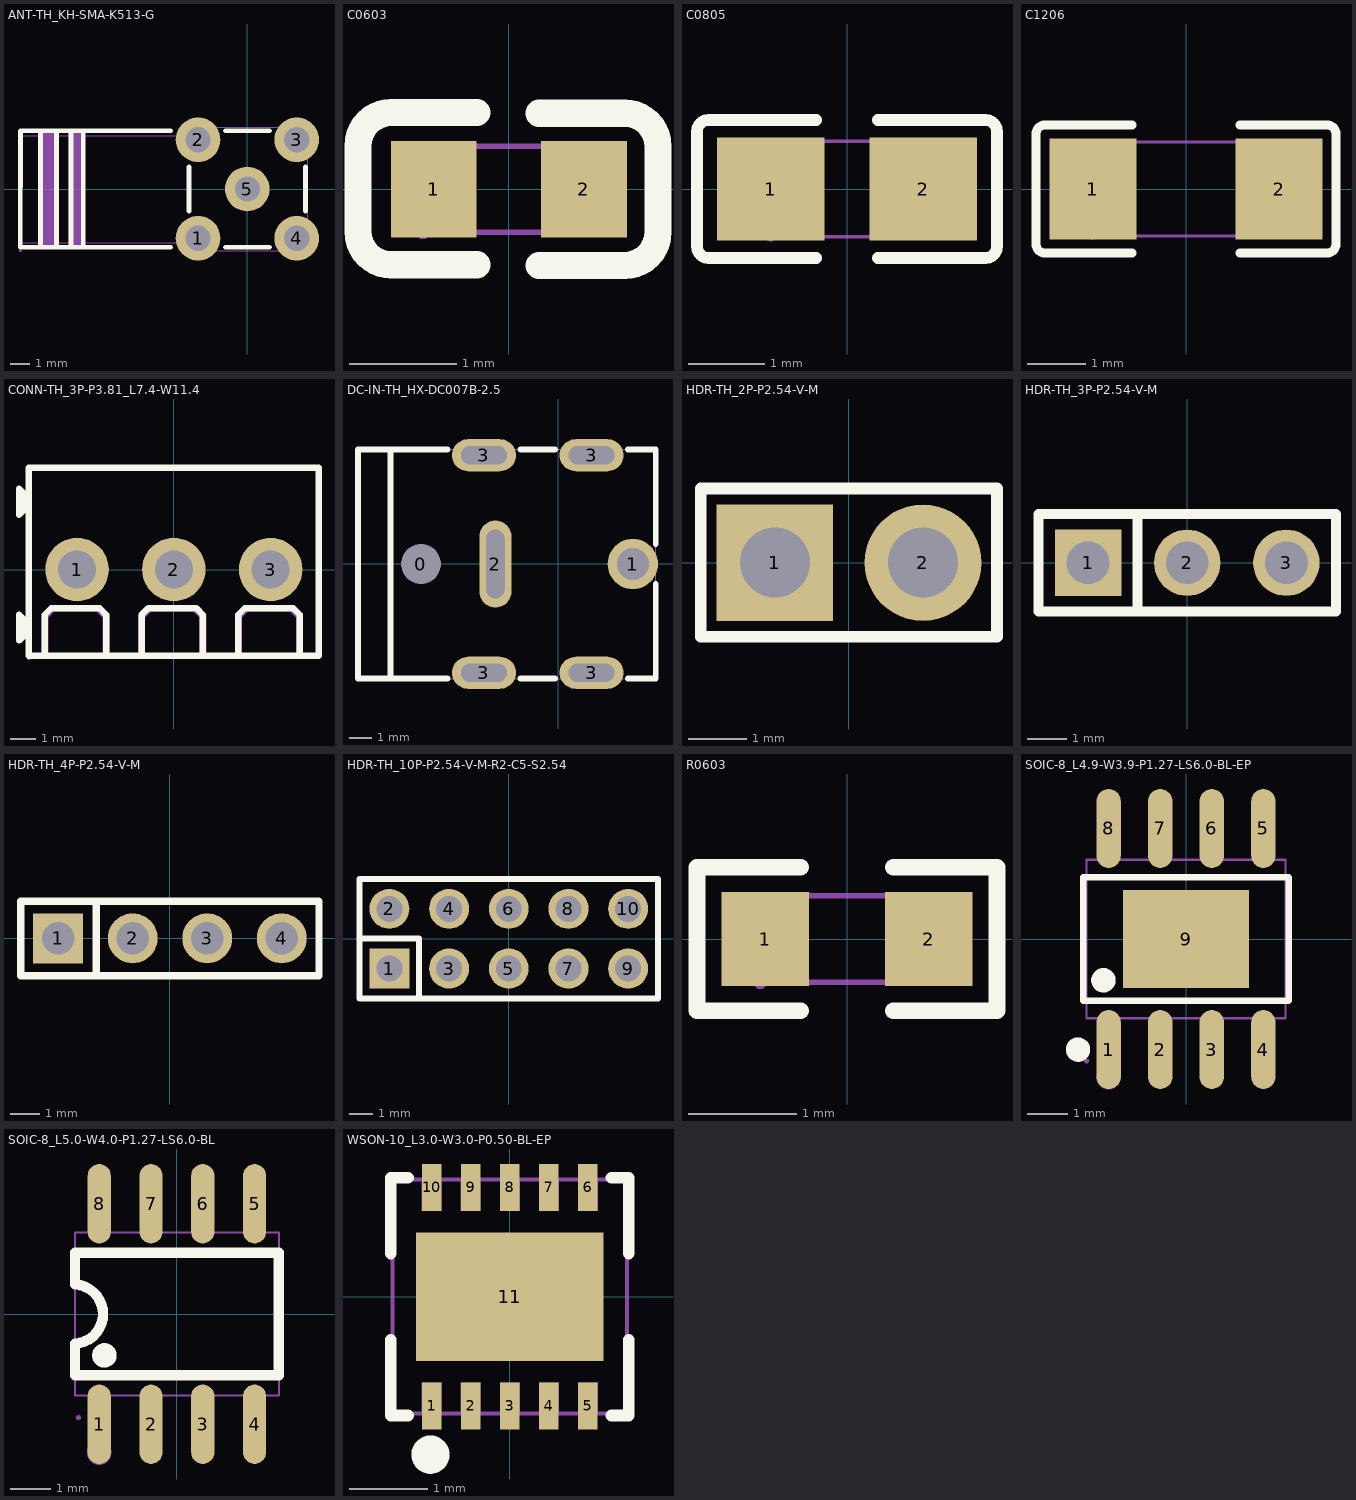
[diagram p0: the footprints below, top view; thin cyan lines are the x and y axes]
# Altium footprint library MISC75514-5.PcbLib: 14 footprints
Each footprint in its own frame and in the unit in brackets; x right, y up, seen from the top. Pads: shape width x height; smd on the part's side, far side on the other; paste and mask are expansions set on the pad; w line width, h text height; cw(c..) or ccw(c..) is an arc to the next point about the centre after c.

## ANT-TH_KH-SMA-K513-G [mm]
height 1.4
pads (5):
  round 2.3 hole 1.3 paste+0.051: 1(-2.54,-2.54) 2(-2.54,2.54) 3(2.54,2.54) 4(2.54,-2.54) 5(0,0)
Top Overlay:
  lines w0.254: -11.69,2.98 -11.7,-2.83 -11.7,-3 -11.5,-3 -3.948,-3 ; -11.69,3 -11.361,3 ; -11.5,3 -3.948,3 ; -10.668,-3 -10.668,3 ; -9.966,3 -9.573,3 ; -9.827,-3 -9.827,3 ; -9.09,-3 -9.09,3 ; -8.595,3 -8.176,3 ; -8.455,-3 -8.455,3 ; -3,-1.132 -3,1.132 ; -1.132,-3 1.132,-3 ; -1.132,3 1.132,3 ; 3,-1.132 3,1.132
Mechanical 2:
  region: -10.64,3 -9.84,3 -9.84,-2.99 -9.85,-3 -10.65,-3
  region: -9.194,2.972 -8.394,2.972 -8.394,-3.018 -8.404,-3.028 -9.204,-3.028
Mechanical 6:
  lines w0.051: -11.7,-2.76 -11.7,2.75 -3.25,2.75 -3.25,3.17 3.1,3.17 3.1,-3.18 -3.25,-3.17 -3.25,-2.76 -11.7,-2.76
Mechanical 8:
  region: -11.635,-3.18 -11.654,-3.226 -11.7,-3.245 -11.746,-3.226 -11.765,-3.18 -11.746,-3.134 -11.7,-3.115 -11.654,-3.134
Mechanical 9:
  region: 0.408,0 0.377,-0.156 0.288,-0.288 0.156,-0.377 0,-0.408 -0.156,-0.377 -0.288,-0.288 -0.377,-0.156 -0.408,0 -0.377,0.156 -0.288,0.288 -0.156,0.377 0,0.408 0.156,0.377 0.288,0.288 0.377,0.156
  region: 2.09,-2.09 2.99,-2.09 2.99,-2.99 2.09,-2.99
  region: -2.99,2.99 -2.09,2.99 -2.09,2.09 -2.99,2.09
  region: 2.09,2.99 2.99,2.99 2.99,2.09 2.09,2.09
  region: -2.99,-2.09 -2.09,-2.09 -2.09,-2.99 -2.99,-2.99

## C0603 [mm]
height 1.4
pads (2):
  rect 0.8x0.9 smd: 1(-0.7,0) 2(0.7,0)
Top Overlay:
  lines w0.254: -0.296,-0.704 -1.096,-0.704 cw(c-1.096,-0.394) -1.406,-0.394 -1.405,0.406 cw(c-1.096,0.406) -1.096,0.715 -0.296,0.715 ; 0.28,-0.71 1.08,-0.71 ccw(c1.08,-0.4) 1.39,-0.4 1.39,0.4 ccw(c1.08,0.4) 1.08,0.71 0.28,0.71
Mechanical 15:
  region: -0.74,-0.4 -0.74,-0.375 -0.775,-0.341 -0.825,-0.341 -0.86,-0.375 -0.86,-0.4 -0.86,-0.425 -0.825,-0.459 -0.776,-0.459 -0.741,-0.425 -0.74,-0.4
  region: 0.8,-0.4 0.8,0.4 0.5,0.4 0.5,-0.4
  region: -0.8,-0.4 -0.8,0.4 -0.5,0.4 -0.5,-0.4
  lines w0.051: -0.8,-0.4 0.8,-0.4 0.8,0.4 -0.8,0.4 -0.8,-0.4

## C0805 [mm]
height 1.4
pads (2):
  rect 1.41x1.35 smd paste-100 mask+0.051: 1(-1,0) 2(1,0)
Top Overlay:
  lines w0.152: -0.401,-0.904 -1.811,-0.904 cw(c-1.811,-0.751) -1.964,-0.751 -1.964,0.751 cw(c-1.811,0.751) -1.811,0.904 -0.401,0.904 ; 0.401,-0.904 1.811,-0.904 ccw(c1.811,-0.751) 1.964,-0.751 1.964,0.751 ccw(c1.811,0.751) 1.811,0.904 0.401,0.904
Top Paste:
  region: 1.705,0.64 1.705,-0.64 1.655,-0.69 0.505,-0.69 0.455,-0.64 0.45,-0.23 0.9,-0.23 0.9,0.22 0.46,0.22 0.455,0.64 0.505,0.69 1.655,0.69
  region: -1.705,-0.64 -1.705,0.64 -1.655,0.69 -0.505,0.69 -0.455,0.64 -0.45,0.23 -0.9,0.23 -0.9,-0.22 -0.46,-0.22 -0.455,-0.64 -0.505,-0.69 -1.655,-0.69
Mechanical 6:
  lines w0.051: -1,-0.625 1,-0.625 1,0.625 -1,0.625 -1,-0.625
Mechanical 8:
  region: -0.935,-0.625 -0.954,-0.671 -1,-0.69 -1.046,-0.671 -1.065,-0.625 -1.046,-0.579 -1,-0.56 -0.954,-0.579
Mechanical 9:
  region: 1,0.625 1,-0.625 0.5,-0.625 0.5,0.625
  region: -1,-0.625 -1,0.625 -0.5,0.625 -0.5,-0.625

## C1206 [mm]
height 1.4
pads (2):
  rect 1.485x1.728 smd paste-100 mask+0.051: 1(-1.593,0) 2(1.593,0)
Top Overlay:
  lines w0.152: -0.926,-1.093 -2.411,-1.093 cw(c-2.411,-0.94) -2.564,-0.94 -2.564,0.94 cw(c-2.411,0.94) -2.411,1.093 -0.926,1.093 ; 0.926,-1.093 2.411,-1.093 ccw(c2.411,-0.94) 2.564,-0.94 2.564,0.94 ccw(c2.411,0.94) 2.411,1.093 0.926,1.093
Top Paste:
  region: -0.85,-0.764 -0.85,-0.394 -0.95,-0.294 -1.255,-0.294 -1.355,-0.194 -1.355,0.194 -1.255,0.294 -0.95,0.294 -0.85,0.394 -0.85,0.764 -0.95,0.864 -2.235,0.864 -2.335,0.764 -2.335,-0.764 -2.235,-0.864 -0.95,-0.864
  region: 0.85,-0.764 0.85,-0.394 0.95,-0.294 1.255,-0.294 1.355,-0.194 1.355,0.194 1.255,0.294 0.95,0.294 0.85,0.394 0.85,0.764 0.95,0.864 2.235,0.864 2.335,0.764 2.335,-0.764 2.235,-0.864 0.95,-0.864
Mechanical 6:
  lines w0.051: -1.6,-0.8 1.6,-0.8 1.6,0.8 -1.6,0.8 -1.6,-0.8
Mechanical 8:
  region: -1.535,-0.8 -1.554,-0.846 -1.6,-0.865 -1.646,-0.846 -1.665,-0.8 -1.646,-0.754 -1.6,-0.735 -1.554,-0.754
Mechanical 9:
  region: 1.6,-0.8 1.6,0.8 1.1,0.8 1.1,-0.8
  region: -1.6,-0.8 -1.6,0.8 -1.1,0.8 -1.1,-0.8

## CONN-TH_3P-P3.81_L7.4-W11.4 [mm]
height 1.4
pads (3):
  round 2.5 hole 1.5 paste+0.051: 1(-3.81,0) 2(0,0) 3(3.81,0)
Top Overlay:
  region: -5.715,2.921 -5.842,2.921 -6.096,3.175 -6.096,2.286 -5.969,2.286 -5.715,2.54
  region: -5.651,-2.095 -5.778,-2.095 -6.032,-1.841 -6.032,-2.73 -5.905,-2.73 -5.651,-2.476
  lines w0.254: -5.715,-2.54 -5.842,-2.54 -6.096,-2.794 -6.096,-1.778 -5.842,-2.032 -5.715,-2.032 ; -5.715,2.413 -5.842,2.413 -6.096,2.159 -6.096,3.175 -5.842,2.921 -5.715,2.921 ; -5.08,-3.302 -5.08,-1.778 -4.826,-1.524 -2.921,-1.524 -2.667,-1.778 -2.667,-3.302 ; -1.27,-3.302 -1.27,-1.778 -1.016,-1.524 0.889,-1.524 1.143,-1.778 1.143,-3.302 ; 2.54,-3.302 2.54,-1.778 2.794,-1.524 4.699,-1.524 4.953,-1.778 4.953,-3.302 ; -5.71,-3.4 5.71,-3.4 5.71,4 -5.71,4 -5.71,-3.4
Mechanical 2:
  region: -5.207,-3.429 -5.207,-1.778 -4.826,-1.397 -2.921,-1.397 -2.54,-1.778 -2.54,-3.429 -2.794,-3.429 -2.794,-1.905 -3.048,-1.651 -4.699,-1.651 -4.953,-1.905 -4.953,-3.429
  region: -1.397,-3.429 -1.397,-1.778 -1.016,-1.397 0.889,-1.397 1.27,-1.778 1.27,-3.429 1.016,-3.429 1.016,-1.905 0.762,-1.651 -0.889,-1.651 -1.143,-1.905 -1.143,-3.429
  region: 2.413,-3.429 2.413,-1.778 2.794,-1.397 4.699,-1.397 5.08,-1.778 5.08,-3.429 4.826,-3.429 4.826,-1.905 4.572,-1.651 2.921,-1.651 2.667,-1.905 2.667,-3.429
Mechanical 6:
  lines w0.051: -5.715,-3.5 -5.715,3.9 5.715,3.9 5.715,-3.5 -5.715,-3.5
Mechanical 8:
  region: -5.65,-3.5 -5.669,-3.546 -5.715,-3.565 -5.761,-3.546 -5.78,-3.5 -5.761,-3.454 -5.715,-3.435 -5.669,-3.454
Mechanical 9:
  region: 3.36,0.3 4.26,0.3 4.26,-0.3 3.36,-0.3
  region: -0.45,0.3 0.45,0.3 0.45,-0.3 -0.45,-0.3
  region: -4.26,0.3 -3.36,0.3 -3.36,-0.3 -4.26,-0.3

## DC-IN-TH_HX-DC007B-2.5 [mm]
height 1.4
pads (7):
  round 1.7 hole 1.7 unplated: 0(-6,0)
  round 2.2 hole 1.4: 1(3.25,0)
  oval 1.4x3.8 hole 0.8 slot 3 at 90 deg: 2(-2.75,0)
  oval 2.8x1.4 hole 0.8 slot 2 at 0 deg: 3(-3.25,-4.75) 3(-3.25,4.75) 3(1.45,-4.75) 3(1.45,4.75)
Top Overlay:
  lines w0.254: -7.325,-5 -7.325,5 ; -4.847,-5 -8.75,-5 -8.75,5 -4.847,5 ; -1.653,-5 -0.147,-5 ; -1.653,5 -0.147,5 ; 3.047,-5 4.25,-5 4.25,-0.877 ; 3.047,5 4.25,5 4.25,0.877
Mechanical 1:
  circle w0.005: c-6,0 r0.85
Mechanical 15:
  region: 3.85,0 3.85,0.119 3.759,0.34 3.59,0.509 3.369,0.6 3.131,0.6 2.91,0.509 2.741,0.34 2.65,0.119 2.65,0 2.65,-0.119 2.741,-0.34 2.91,-0.509 3.131,-0.6 3.369,-0.6 3.59,-0.509 3.759,-0.34 3.85,-0.119 3.85,0
  region: -2.65,-0.8 -2.85,-0.8 -2.85,0.8 -2.65,0.8
  region: 0.65,-4.9 0.65,-4.6 2.25,-4.6 2.25,-4.9
  region: -4.05,-4.9 -4.05,-4.6 -2.45,-4.6 -2.45,-4.9
  region: 0.65,4.6 0.65,4.9 2.25,4.9 2.25,4.6
  region: -4.05,4.6 -4.05,4.9 -2.45,4.9 -2.45,4.6
  region: 4.31,-5 4.309,-4.976 4.274,-4.943 4.226,-4.943 4.191,-4.976 4.19,-5 4.191,-5.024 4.226,-5.058 4.274,-5.058 4.309,-5.024 4.31,-5
  lines w0.051: -8.75,-5 -8.75,5 4.25,5 4.25,-5 -8.75,-5

## HDR-TH_2P-P2.54-V-M [mm]
height 1.4
pads (2):
  rect 2x2 hole 1.2 paste+0.051: 1(-1.27,0)
  round 2 hole 1.2 paste+0.051: 2(1.27,0)
Top Overlay:
  lines w0.203: -2.54,-1.27 -2.54,1.27 -0.635,1.27 2.54,1.27 2.54,-1.27 -2.54,-1.27
Mechanical 6:
  lines w0.051: -2.54,-1.25 2.54,-1.25 2.54,1.25 -2.54,1.25 -2.54,-1.25
Mechanical 8:
  region: -2.475,-1.25 -2.494,-1.296 -2.54,-1.315 -2.586,-1.296 -2.605,-1.25 -2.586,-1.204 -2.54,-1.185 -2.494,-1.204
Mechanical 9:
  region: -1.59,0.32 -0.95,0.32 -0.95,-0.32 -1.59,-0.32
  region: 0.95,0.32 1.59,0.32 1.59,-0.32 0.95,-0.32

## HDR-TH_3P-P2.54-V-M [mm]
height 1.4
pads (3):
  rect 1.7x1.7 hole 1.1 paste+0.051: 1(-2.54,0)
  round 1.7 hole 1.1 paste+0.051: 2(0,0) 3(2.54,0)
Top Overlay:
  lines w0.254: -1.27,-1.25 -1.27,1.25 ; 3.809,-1.25 3.809,1.25 -3.81,1.25 -3.81,-1.25 3.81,-1.25
Mechanical 6:
  lines w0.051: -3.81,-1.25 3.81,-1.25 3.81,1.25 -3.81,1.25 -3.81,-1.25
Mechanical 8:
  region: -3.745,-1.25 -3.764,-1.296 -3.81,-1.315 -3.856,-1.296 -3.875,-1.25 -3.856,-1.204 -3.81,-1.185 -3.764,-1.204
Mechanical 9:
  region: -2.86,0.32 -2.22,0.32 -2.22,-0.32 -2.86,-0.32
  region: -0.32,0.32 0.32,0.32 0.32,-0.32 -0.32,-0.32
  region: 2.22,0.32 2.86,0.32 2.86,-0.32 2.22,-0.32

## HDR-TH_4P-P2.54-V-M [mm]
height 1.4
pads (4):
  rect 1.7x1.7 hole 1.1 paste+0.051: 1(-3.81,0)
  round 1.7 hole 1.1 paste+0.051: 2(-1.27,0) 3(1.27,0) 4(3.81,0)
Top Overlay:
  lines w0.254: -2.516,-1.27 -2.516,1.27 ; -2.516,1.27 -5.08,1.27 -5.08,-1.27 5.08,-1.27 5.08,1.27 -2.516,1.27
Mechanical 6:
  lines w0.051: -5.08,-1.25 5.08,-1.25 5.08,1.25 -5.08,1.25 -5.08,-1.25
Mechanical 8:
  region: -5.015,-1.25 -5.034,-1.296 -5.08,-1.315 -5.126,-1.296 -5.145,-1.25 -5.126,-1.204 -5.08,-1.185 -5.034,-1.204
Mechanical 9:
  region: 3.49,0.32 4.13,0.32 4.13,-0.32 3.49,-0.32
  region: 0.95,0.32 1.59,0.32 1.59,-0.32 0.95,-0.32
  region: -1.59,0.32 -0.95,0.32 -0.95,-0.32 -1.59,-0.32
  region: -4.13,0.32 -3.49,0.32 -3.49,-0.32 -4.13,-0.32

## HDR-TH_10P-P2.54-V-M-R2-C5-S2.54 [mm]
height 1.4
pads (10):
  rect 1.7x1.7 hole 1.1 paste+0.051: 1(-5.08,-1.27)
  round 1.7 hole 1.1 paste+0.051: 2(-5.08,1.27) 3(-2.54,-1.27) 4(-2.54,1.27) 5(0,-1.27) 6(0,1.27) 7(2.54,-1.27) 8(2.54,1.27) 9(5.08,-1.27) 10(5.08,1.27)
Top Overlay:
  lines w0.254: -6.35,0 -3.81,0.007 -3.81,-2.54 ; -6.35,-2.54 6.35,-2.54 6.35,2.54 -6.35,2.54 -6.35,-2.54
Mechanical 6:
  lines w0.051: -6.35,-2.5 -6.35,2.5 6.35,2.5 6.35,-2.5 -6.35,-2.5
Mechanical 8:
  region: -6.285,-2.5 -6.304,-2.546 -6.35,-2.565 -6.396,-2.546 -6.415,-2.5 -6.396,-2.454 -6.35,-2.435 -6.304,-2.454
Mechanical 9:
  region: -5.4,1.59 -4.76,1.59 -4.76,0.95 -5.4,0.95
  region: -5.4,-0.95 -4.76,-0.95 -4.76,-1.59 -5.4,-1.59
  region: -2.86,1.59 -2.22,1.59 -2.22,0.95 -2.86,0.95
  region: -2.86,-0.95 -2.22,-0.95 -2.22,-1.59 -2.86,-1.59
  region: -0.32,1.59 0.32,1.59 0.32,0.95 -0.32,0.95
  region: -0.32,-0.95 0.32,-0.95 0.32,-1.59 -0.32,-1.59
  region: 2.22,1.59 2.86,1.59 2.86,0.95 2.22,0.95
  region: 2.22,-0.95 2.86,-0.95 2.86,-1.59 2.22,-1.59
  region: 4.76,1.59 5.4,1.59 5.4,0.95 4.76,0.95
  region: 4.76,-0.95 5.4,-0.95 5.4,-1.59 4.76,-1.59

## R0603 [mm]
height 1.4
pads (2):
  rect 0.806x0.864 smd paste-100 mask+0.051: 1(-0.753,0) 2(0.753,0)
Top Overlay:
  lines w0.152: -0.426,-0.661 -1.385,-0.661 -1.385,0.661 -0.426,0.661 ; 0.426,-0.661 1.385,-0.661 1.385,0.661 0.426,0.661
Top Paste:
  region: -0.355,0.4 -0.355,0.172 -0.735,0.172 -0.735,-0.158 -0.355,-0.158 -0.355,-0.4 -0.405,-0.45 -1.195,-0.45 -1.245,-0.4 -1.245,0.4 -1.195,0.45 -0.405,0.45
  region: 1.195,0.45 0.395,0.45 0.345,0.4 0.345,0.172 0.715,0.172 0.715,-0.158 0.345,-0.158 0.345,-0.4 0.395,-0.45 1.195,-0.45 1.245,-0.4 1.245,0.4
Mechanical 15:
  region: -0.74,-0.4 -0.741,-0.376 -0.776,-0.342 -0.824,-0.342 -0.859,-0.376 -0.86,-0.4 -0.859,-0.424 -0.825,-0.458 -0.776,-0.458 -0.741,-0.424 -0.74,-0.4
  region: 0.8,-0.4 0.8,0.4 0.5,0.4 0.5,-0.4
  region: -0.8,-0.4 -0.8,0.4 -0.5,0.4 -0.5,-0.4
  lines w0.051: -0.8,-0.4 0.8,-0.4 0.8,0.4 -0.8,0.4 -0.8,-0.4

## SOIC-8_L4.9-W3.9-P1.27-LS6.0-BL-EP [mm]
height 1.4
pads (9):
  oval 0.602x1.941 smd paste+0.051: 1(-1.905,-2.721) 2(-0.635,-2.721) 3(0.635,-2.721) 4(1.905,-2.721) 5(1.905,2.721) 6(0.635,2.721) 7(-0.635,2.721) 8(-1.905,2.721)
  rect 3.098x2.41 smd paste+0.051: 9(0,0)
Top Overlay:
  circle w0.3: c-2.658,-2.721 r0.15
  circle w0.3: c-2.032,-1.016 r0.15
  lines w0.152: -2.526,-1.521 2.526,-1.521 2.526,1.521 -2.526,1.521 -2.526,-1.521
Mechanical 2:
  circle w0.3: c-1.905,-3.4 r0.15
Mechanical 6:
  lines w0.051: -2.45,-1.95 2.45,-1.95 2.45,1.95 -2.45,1.95 -2.45,-1.95
Mechanical 7:
  region: 1.69,2.36 1.69,1.94 2.12,1.94 2.12,2.36
  region: 0.42,2.36 0.42,1.94 0.85,1.94 0.85,2.36
  region: -0.85,2.36 -0.85,1.94 -0.42,1.94 -0.42,2.36
  region: -2.12,2.36 -2.12,1.94 -1.69,1.94 -1.69,2.36
  region: 1.69,-2.36 1.69,-1.94 2.12,-1.94 2.12,-2.36
  region: 0.42,-2.36 0.42,-1.94 0.85,-1.94 0.85,-2.36
  region: -0.85,-2.36 -0.85,-1.94 -0.42,-1.94 -0.42,-2.36
  region: -2.12,-2.36 -2.12,-1.94 -1.69,-1.94 -1.69,-2.36
Mechanical 8:
  region: -2.385,-3 -2.404,-3.046 -2.45,-3.065 -2.496,-3.046 -2.515,-3 -2.496,-2.954 -2.45,-2.935 -2.404,-2.954
Mechanical 9:
  region: -1.549,1.205 1.549,1.205 1.549,-1.205 -1.549,-1.205
  region: 1.69,3 1.69,2.35 2.12,2.35 2.12,3
  region: 0.42,3 0.42,2.35 0.85,2.35 0.85,3
  region: -0.85,3 -0.85,2.35 -0.42,2.35 -0.42,3
  region: -2.12,3 -2.12,2.35 -1.69,2.35 -1.69,3
  region: 1.69,-3 1.69,-2.35 2.12,-2.35 2.12,-3
  region: 0.42,-3 0.42,-2.35 0.85,-2.35 0.85,-3
  region: -0.85,-3 -0.85,-2.35 -0.42,-2.35 -0.42,-3
  region: -2.12,-3 -2.12,-2.35 -1.69,-2.35 -1.69,-3

## SOIC-8_L5.0-W4.0-P1.27-LS6.0-BL [mil]
height 55.12
pads (8):
  oval 22.38x76.78 smd paste+2: 1(-75,-106.5) 2(-25,-106.5) 3(25,-106.5) 4(75,-106.5) 5(75,106.5) 6(25,106.5) 7(-25,106.5) 8(-75,106.5)
Top Overlay:
  circle w11.81: c-70,-40 r5.91
  lines w10: -98.43,-28.61 ccw(c-99.99,0) -98.23,28.59 ; -98.42,-28.61 -98.42,-59.05 98.42,-59.05 98.42,59.05 -98.42,59.05 -98.42,28.59
Mechanical 2:
  circle w11.81: c-75,-133.86 r5.91
Mechanical 6:
  lines w2: -98.42,-78.74 98.42,-78.74 98.42,78.74 -98.42,78.74 -98.42,-78.74
Mechanical 7:
  region: -83.07,-85.63 -83.07,-76.38 -66.93,-76.38 -66.93,-85.63
  region: -33.07,-85.63 -33.07,-76.38 -16.93,-76.38 -16.93,-85.63
  region: 16.93,-85.63 16.93,-76.38 33.07,-76.38 33.07,-85.63
  region: 66.93,-85.63 66.93,-76.38 83.07,-76.38 83.07,-85.63
  region: -83.07,76.38 -83.07,85.63 -66.93,85.63 -66.93,76.38
  region: -33.07,76.38 -33.07,85.63 -16.93,85.63 -16.93,76.38
  region: 16.93,76.38 16.93,85.63 33.07,85.63 33.07,76.38
  region: 66.93,76.38 66.93,85.63 83.07,85.63 83.07,76.38
Mechanical 8:
  region: -92.44,-100 -93.19,-101.81 -95,-102.56 -96.81,-101.81 -97.56,-100 -96.81,-98.19 -95,-97.44 -93.19,-98.19
Mechanical 9:
  region: -83.07,-118.11 -83.07,-85.24 -66.93,-85.24 -66.93,-118.11
  region: -33.07,-118.11 -33.07,-85.24 -16.93,-85.24 -16.93,-118.11
  region: 16.93,-118.11 16.93,-85.24 33.07,-85.24 33.07,-118.11
  region: 66.93,-118.11 66.93,-85.24 83.07,-85.24 83.07,-118.11
  region: -83.07,85.24 -83.07,118.11 -66.93,118.11 -66.93,85.24
  region: -33.07,85.24 -33.07,118.11 -16.93,118.11 -16.93,85.24
  region: 16.93,85.24 16.93,118.11 33.07,118.11 33.07,85.24
  region: 66.93,85.24 66.93,118.11 83.07,118.11 83.07,85.24

## WSON-10_L3.0-W3.0-P0.50-BL-EP [mm]
height 1.4
pads (11):
  rect 0.25x0.6 smd paste+0.051: 1(-1.001,-1.4) 2(-0.5,-1.4) 3(0,-1.4) 4(0.5,-1.4) 5(1.001,-1.4) 6(1.001,1.4) 7(0.5,1.4) 8(0,1.4) 9(-0.5,1.4) 10(-1.001,1.4)
  rect 2.4x1.65 smd paste+0.051: 11(0,0)
Top Overlay:
  lines w0.15: -1.524,-0.554 -1.524,-1.524 -1.305,-1.524 ; -1.524,0.554 -1.524,1.524 -1.305,1.524 ; 1.305,-1.524 1.524,-1.524 1.524,-0.554 ; 1.305,1.524 1.524,1.524 1.524,0.554
  lines w0.25: -1.019,-1.905 ccw(c-1.017,-2.025) -1.016,-1.905
Mechanical 6:
  lines w0.051: -1.5,-1.5 -1.5,1.5 1.5,1.5 1.5,-1.5 -1.5,-1.5
Mechanical 8:
  region: -1.439,-1.502 -1.458,-1.548 -1.504,-1.567 -1.55,-1.548 -1.569,-1.502 -1.55,-1.456 -1.504,-1.437 -1.458,-1.456
Mechanical 9:
  region: -1.126,1.501 -0.876,1.501 -0.876,1.101 -1.126,1.101
  region: -0.625,1.501 -0.375,1.501 -0.375,1.101 -0.625,1.101
  region: -0.125,1.501 0.125,1.501 0.125,1.101 -0.125,1.101
  region: 0.375,1.501 0.625,1.501 0.625,1.101 0.375,1.101
  region: 0.876,1.501 1.126,1.501 1.126,1.101 0.876,1.101
  region: -0.876,-1.501 -1.126,-1.501 -1.126,-1.101 -0.876,-1.101
  region: -0.375,-1.501 -0.625,-1.501 -0.625,-1.101 -0.375,-1.101
  region: 0.125,-1.501 -0.125,-1.501 -0.125,-1.101 0.125,-1.101
  region: 0.625,-1.501 0.375,-1.501 0.375,-1.101 0.625,-1.101
  region: 1.126,-1.501 0.876,-1.501 0.876,-1.101 1.126,-1.101